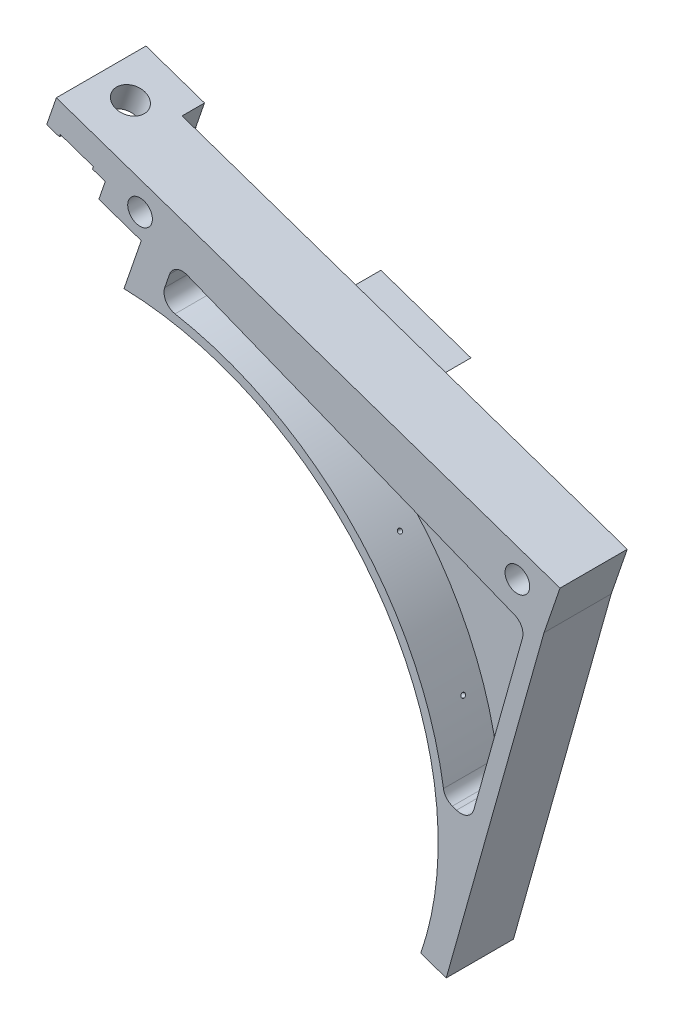
SolidWorks part; units mm, degrees
ref_plane "前视基准面" through (0, 0, 0) normal (0, 0, 1) x (1, 0, 0)
ref_plane "上视基准面" through (0, 0, 0) normal (0, 1, 0) x (1, 0, 0)
ref_plane "右视基准面" through (0, 0, 0) normal (1, 0, 0) x (0, 0, -1)
sketch "草图1" plane through (0, 0, 0) normal (0, 0, 1) x (1, 0, 0)
  line L0 (-181.8738, 171.3731) -> (-174.9089, 177.4414) construction
  line L1 (-174.9089, 177.4414) -> (-194.9973, 184.333) construction
  line L2 (-194.9973, 184.333) -> (-193.2244, 175.2671) construction
  line L3 (-181.8738, 171.3731) -> (-174.9089, 177.4414)
  line L4 (-174.9089, 177.4414) -> (-194.9973, 184.333)
  line L5 (-194.9973, 184.333) -> (-193.2244, 175.2671)
  line L6 (-193.2244, 175.2671) -> (-181.8738, 171.3731)
extrude "凸台-拉伸1" add sketch "草图1" against normal up to surface (8 mm away)
sketch "草图2" plane through (0, 0, 0) normal (0, 0, 1) x (1, 0, 0)
  line L0 (-132.0344, 165.9043) -> (-231.3524, 199.9768)
  line L1 (-123.2729, 191.4432) -> (-135.6039, 155.4995) construction
  line L2 (-234.9219, 189.572) -> (-222.5909, 225.5157) construction
  line L3 (-135.6039, 155.4995) -> (-181.8738, 171.3731) construction
  line L4 (-132.0344, 165.9043) -> (-135.6039, 155.4995)
  line L5 (-234.9219, 189.572) -> (-231.3524, 199.9768)
  line L6 (-157.4248, 77.8738) -> (-168.7773, 81.7623)
  line L8 (-293.6552, 124.5352) -> (-305.0078, 128.4236)
  line L9 (-135.6039, 155.4995) -> (-157.4248, 77.8738)
  line L10 (-234.9219, 189.572) -> (-267.9216, 171.9726)
  circle A0 centre (-231.2163, 103.1487) radius 66 construction
  arc A1 (-168.7773, 81.7623) -> (-293.6552, 124.5352) centre (-231.2163, 103.1487) ccw
  arc A2 (-157.4248, 77.8738) -> (-155.0636, 86.2737) centre (-231.2163, 103.1487) ccw
  arc A3 (-267.9216, 171.9726) -> (-305.0078, 128.4236) centre (-231.2163, 103.1487) ccw
  circle A4 centre (-225.7323, 191.7055) radius 2.75
  arc A5 (-157.4248, 77.8738) -> (-305.0078, 128.4236) centre (-231.2163, 103.1487) ccw construction
  circle A6 centre (-141.5485, 162.825) radius 2.75
  line M2 (-193.2244, 175.2671) -> (-181.8738, 171.3731)
  line M3 (-181.8738, 171.3731) -> (-174.9089, 177.4414)
  line M4 (-174.9089, 177.4414) -> (-194.9973, 184.333)
  line M5 (-194.9973, 184.333) -> (-193.2244, 175.2671)
  dimension "D2" = 5.5
  dimension "D3" = 5.5
  dimension "D1" = 11
extrude "凸台-拉伸2" add sketch "草图2" along normal blind 15 separate body contours L10 A3 L8 A1 L6 L9 L4 L0 L5 A6 A4 M2 M5 M4 M3
sketch "草图4" plane through (0, 0, 15) normal (0, 0, 1) x (1, 0, 0)
  line L2 (-207.8856, 171.2639) -> (-296.9833, 201.7814)
  line L3 (-296.9833, 201.7814) -> (-325.4692, 118.6151)
  line L4 (-325.4692, 118.6151) -> (-168.2563, 64.767)
  line L5 (-163.1011, 79.8181) -> (-168.2563, 64.767)
  arc A2 (-163.1011, 79.8181) -> (-207.8856, 171.2639) centre (-231.2163, 103.1487) ccw
  point P0 (-231.2163, 103.1487)
  point P1 (-168.7773, 81.7623)
  point P2 (-293.6552, 124.5352)
  point P5 (-299.3315, 126.4794)
extrude "切除-拉伸1" cut sketch "草图4" against normal blind 15
sketch "草图5" plane through (0, 0, 15) normal (0, 0, 1) x (1, 0, 0)
  line L0 (-234.9219, 189.572) -> (-225.4631, 186.327)
  line L2 (-225.4631, 186.327) -> (-228.267, 178.154)
  line L3 (-237.7258, 181.399) -> (-228.267, 178.154)
  line L4 (-234.9219, 189.572) -> (-251.1939, 195.1544)
  line L5 (-251.1939, 195.1544) -> (-253.9978, 186.9813)
  line L6 (-253.9978, 186.9813) -> (-237.7258, 181.399)
  dimension "D1" = 10
extrude "切除-拉伸2" cut sketch "草图5" against normal blind 8
sketch "草图6" plane through (0, 0, 7) normal (0, 0, 1) x (1, 0, 0)
  line L0 (-234.9219, 189.572) -> (-237.6955, 181.4743)
  line L1 (-245.2522, 184.0626) -> (-228.239, 178.2353) construction
  line L2 (-237.6955, 181.4743) -> (-249.3797, 185.4764)
  line L3 (-249.3797, 185.4764) -> (-246.6061, 193.5741)
  line L4 (-246.6061, 193.5741) -> (-234.9219, 189.572)
extrude "切除-拉伸3" cut sketch "草图6" against normal through all
sketch "草图7" plane through (0, 0, 7) normal (0, 0, 1) x (1, 0, 0)
  line L0 (-226.851, 182.2812) -> (-236.3087, 185.5232) construction
  line L1 (-228.239, 178.2353) -> (-225.4631, 186.327) construction
  line L2 (-237.6955, 181.4743) -> (-234.9219, 189.572) construction
  circle A0 centre (-231.5799, 183.9022) radius 0.5
  dimension "D1" = 1
extrude "切除-拉伸4" cut sketch "草图7" against normal through all
sketch "草图8" plane through (0, 0, 15) normal (0, 0, 1) x (1, 0, 0)
  line L0 (-229.3066, 175.1234) -> (-227.0823, 181.6071) construction
  line L1 (-207.8856, 171.2639) -> (-228.239, 178.2353) construction
  line L2 (-229.3066, 175.1234) -> (-228.239, 178.2353)
  line L3 (-207.8856, 171.2639) -> (-228.239, 178.2353)
  arc A0 (-207.8856, 171.2639) -> (-229.3066, 175.1234) centre (-231.2163, 103.1487) ccw
extrude "凸台-拉伸3" add sketch "草图8" against normal up to surface (15 mm away) up to face at (-231.0799, 183.9022, 0)
sketch "草图9" plane through (35.0724, 102.2326, 0) normal (0.3245, 0.9459, 0) x (0.9459, -0.3245, 0)
  line L0 (-294.5254, 5) -> (-283.7254, 5)
  line L1 (-294.5254, 5) -> (-294.5254, -15)
  line L2 (-283.7254, 5) -> (-283.7254, -15)
  line L3 (-294.5254, -15) -> (-283.7254, -15)
  line L4 (-178.7254, -15) -> (-283.7254, -15) construction
  line L5 (-283.7254, -15) -> (-283.7254, 0) construction
  dimension "D1" = 0
  dimension "D2" = 0
extrude "凸台-拉伸4" add sketch "草图9" along normal up to surface (6 mm away) up to face at (-181.6934, 182.9405, 7.5)
sketch "草图10" plane through (0, 0, 15) normal (0, 0, 1) x (1, 0, 0)
  line L0 (-236.3318, 194.7074) -> (-236.1371, 195.275)
  line L1 (-236.3318, 194.7074) -> (-233.45, 193.7188)
  line L2 (-236.1371, 195.275) -> (-233.2553, 194.2864)
  line L3 (-233.45, 193.7188) -> (-233.2553, 194.2864)
  line L4 (-243.515, 197.8061) -> (-233.2994, 194.3015) construction
  line L5 (-236.1371, 195.275) -> (-236.3318, 194.7074) construction
  line L6 (-243.7097, 197.2385) -> (-246.5473, 198.212)
  line L7 (-243.7097, 197.2385) -> (-241.568, 203.4814)
  line L8 (-246.5473, 198.212) -> (-244.4056, 204.4549)
  line L9 (-241.568, 203.4814) -> (-244.4056, 204.4549)
  line L10 (-132.0344, 165.9043) -> (-241.568, 203.4814) construction
  dimension "D1" = 0
extrude "凸台-拉伸5" add sketch "草图10" against normal up to surface (20 mm away) up to face at (-237.4337, 198.8914, -5)
hole_wizard "Ø1.0 (1) 直径孔1" positions "草图11" profile "草图12" hole size "Ø1.0" standard "GB" end condition through all
sketch "草图11" plane through (35.0724, 102.2326, 0) normal (-0.3245, -0.9459, 0) x (-0.9459, 0.3245, 0)
  point P0 (290.6254, -5)
sketch "草图12" plane through (-239.826, 196.5405, 5) normal (0, 0, 1) x (0.9459, -0.3245, 0)
  line L0 (0, 0) -> (0, 42.4645)
  line L1 (0, 42.4645) -> (3.25, 42.4645)
  line L2 (3.25, 42.4645) -> (3.25, 0)
  line L5 (3.25, 0) -> (0, 0)
  line L11 (0, -6.35) -> (0, 107.95) construction
  dimension "通孔孔直径" = 6.5
  dimension "通孔孔深度" = 42.4645
sketch "草图13" plane through (0, 0, 0) normal (0, 0, 1) x (1, 0, 0)
  line L4 (-193.2244, 175.2671) -> (-181.8738, 171.3731)
  line L5 (-181.8738, 171.3731) -> (-174.9089, 177.4414)
  line L6 (-174.9089, 177.4414) -> (-194.9973, 184.333)
  line L7 (-194.9973, 184.333) -> (-193.2244, 175.2671)
  line L8 (-193.2244, 175.2671) -> (-181.8738, 171.3731)
  line L9 (-181.8738, 171.3731) -> (-174.9089, 177.4414)
  line L10 (-174.9089, 177.4414) -> (-194.9973, 184.333)
  line L11 (-194.9973, 184.333) -> (-193.2244, 175.2671)
  dimension "D1" = 0
extrude "凸台-拉伸6" add sketch "草图13" along normal up to surface (15 mm away) up to face at (-209.8483, 173.4501, 15)
sketch "草图14" plane through (0, 0, 15) normal (0, 0, 1) x (1, 0, 0)
  line L0 (-156.0478, 111.7742) -> (-155.1207, 111.4561)
  line L1 (-220.2209, 179.8695) -> (-219.157, 182.9708)
  line L2 (-151.2591, 113.482) -> (-140.4123, 152.0686)
  line L3 (-215.2081, 184.7839) -> (-142.1891, 155.6671)
  arc A0 (-163.1011, 79.8181) -> (-229.3066, 175.1234) centre (-231.2163, 103.1487) ccw construction
  arc A1 (-163.1011, 79.8181) -> (-229.3066, 175.1234) centre (-231.2163, 103.1487) ccw
  arc A2 (-158.0409, 114.1653) -> (-217.9222, 175.9448) centre (-231.2163, 103.1487) ccw
  arc A3 (-217.9222, 175.9448) -> (-220.2209, 179.8695) centre (-217.3832, 178.896) cw
  arc A4 (-161.209, 79.17) -> (-229.2536, 177.1227) centre (-231.2163, 103.1487) ccw construction
  arc A5 (-219.157, 182.9708) -> (-215.2081, 184.7839) centre (-216.3193, 181.9973) cw
  arc A6 (-142.1891, 155.6671) -> (-140.4123, 152.0686) centre (-143.3003, 152.8805) cw
  arc A7 (-155.1207, 111.4561) -> (-151.2591, 113.482) centre (-154.1472, 114.2938) ccw
  arc A8 (-156.0478, 111.7742) -> (-158.0409, 114.1653) centre (-155.0743, 114.6119) cw
  point P13 (-221.3796, 176.492)
  point P16 (-218.1346, 185.9509)
  point P21 (-152.1181, 110.4261)
  point P24 (-157.7935, 112.3731)
  dimension "D3" = 3
  dimension "D1" = 6
  dimension "D2" = 10
extrude "切除-拉伸5" cut sketch "草图14" against normal blind 12 contours A8 L0 A7 L2 A6 L3 A5 L1 A3 A2
ref_plane "基准面4" through (0, 0, 7.5) normal (0, 0, 1) x (1, 0, 0)
sketch "草图15" plane through (0, 0, 7.5) normal (0, 0, 1) x (1, 0, 0)
  line L0 (-205.4487, 166.6766) -> (-201.7725, 175.7402)
  line L1 (-204.9854, 166.4887) -> (-201.3091, 175.5523)
  line L2 (-201.3091, 175.5523) -> (-201.7725, 175.7402)
  line L3 (-204.9854, 166.4887) -> (-205.4487, 166.6766)
  line L5 (-230.7529, 102.9608) -> (-201.3091, 175.5523) construction
  line L6 (-231.2163, 103.1487) -> (-201.7725, 175.7402) construction
revolve "切除-旋转1" cut sketch "草图15" angle 360 about L0
sketch "草图16" plane through (0, 0, 7.5) normal (0, 0, 1) x (1, 0, 0)
  line L0 (-177.8731, 149.2772) -> (-169.2628, 156.723)
  line L1 (-177.5461, 148.899) -> (-168.9357, 156.3448)
  line L2 (-169.2628, 156.723) -> (-168.9357, 156.3448)
  line L3 (-177.8731, 149.2772) -> (-177.5461, 148.899)
  line L5 (-231.2163, 103.1487) -> (-169.2628, 156.723) construction
  line L6 (-230.8892, 102.7705) -> (-168.9357, 156.3448) construction
revolve "切除-旋转2" cut sketch "草图16" angle 360 about L0
sketch "草图17" plane through (0, 0, 7.5) normal (0, 0, 1) x (1, 0, 0)
  line L0 (-166.3617, 125.1094) -> (-154.938, 128.9777)
  line L1 (-166.2013, 124.6358) -> (-154.7777, 128.5041)
  line L2 (-166.3617, 125.1094) -> (-166.2013, 124.6358)
  line L3 (-154.938, 128.9777) -> (-154.7777, 128.5041)
  line L4 (-154.7777, 128.5041) -> (-154.7955, 128.3663)
  line L6 (-231.2163, 103.1487) -> (-154.938, 128.9777) construction
  line L7 (-231.0559, 102.6751) -> (-154.7777, 128.5041) construction
revolve "切除-旋转3" cut sketch "草图17" angle 360 about L0
hole_wizard "M3 螺纹孔1" positions "草图18" profile "草图19" tap size "M3" standard "GB" end condition through all
sketch "草图18" plane through (0, 0, 7) normal (0, 0, 1) x (1, 0, 0)
  point P0 (-231.5799, 183.9022)
sketch "草图19" plane through (-231.5799, 183.9022, 7) normal (1, 0, 0) x (0, -1, 0)
  line L0 (0, 0) -> (0, 15)
  line L1 (0, 15) -> (1.25, 15)
  line L2 (1.25, 15) -> (1.25, 0)
  line L5 (1.25, 0) -> (0, 0)
  line L11 (0, -6.35) -> (0, 107.95) construction
  dimension "通孔螺纹孔钻头直径" = 2.5
  dimension "通孔螺纹孔钻头深度" = 15
cosmetic thread "孔螺蚊线1" parameters "D2"=3
